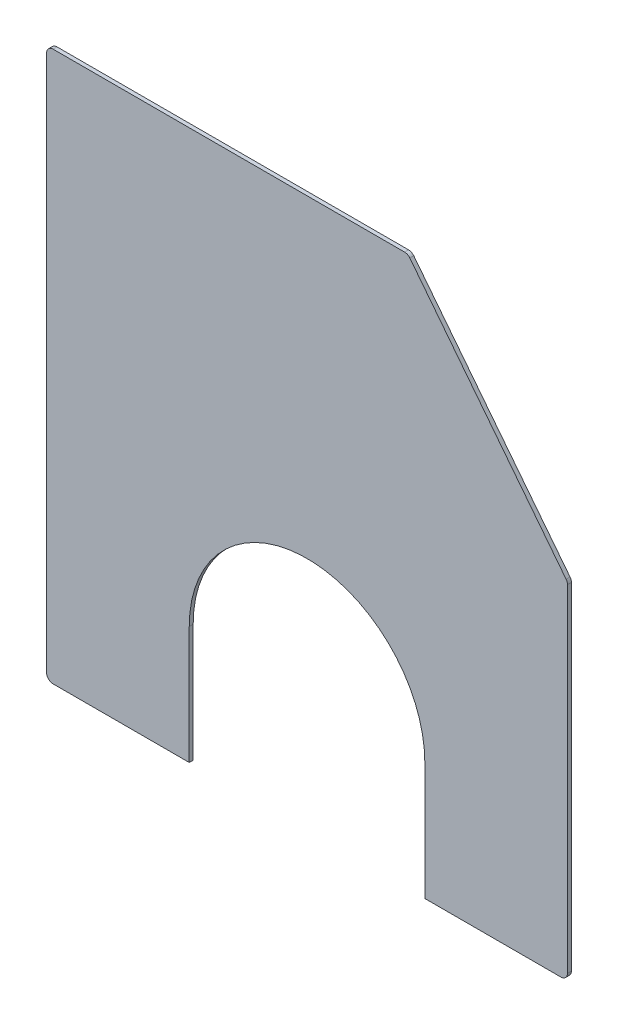
from build123d import *

# Parameters (mm, degrees)
BOSS_EXTRUDE1_DEPTH = 3


with BuildPart() as part:
    # Sketch1 → Boss-Extrude1 (new body)
    with BuildSketch(Plane.XY):
        with BuildLine():
            Line((0, 5), (0, 415))
            ThreePointArc((0, 415), (1.464466094, 418.535533906), (5, 420))
            Line((5, 420), (273.602650759, 420))
            ThreePointArc((273.602650759, 420), (275.794506493, 419.493970231), (277.542704528, 418.078307377))
            Line((277.542704528, 418.078307377), (396.940053768, 265.25666931))
            ThreePointArc((396.940053768, 265.25666931), (397.727592878, 263.806202706), (398, 262.178361934))
            Line((398, 262.178361934), (398, 5))
            ThreePointArc((398, 5), (396.535533906, 1.464466094), (393, 0))
            Line((393, 0), (289, 0))
            Line((289, 0), (289, 90))
            ThreePointArc((289, 90), (199, 180), (109, 90))
            Line((109, 90), (109, 0))
            Line((109, 0), (5, 0))
            ThreePointArc((5, 0), (1.464466094, 1.464466094), (0, 5))
        make_face()
    extrude(amount=BOSS_EXTRUDE1_DEPTH)


solid = part.part
